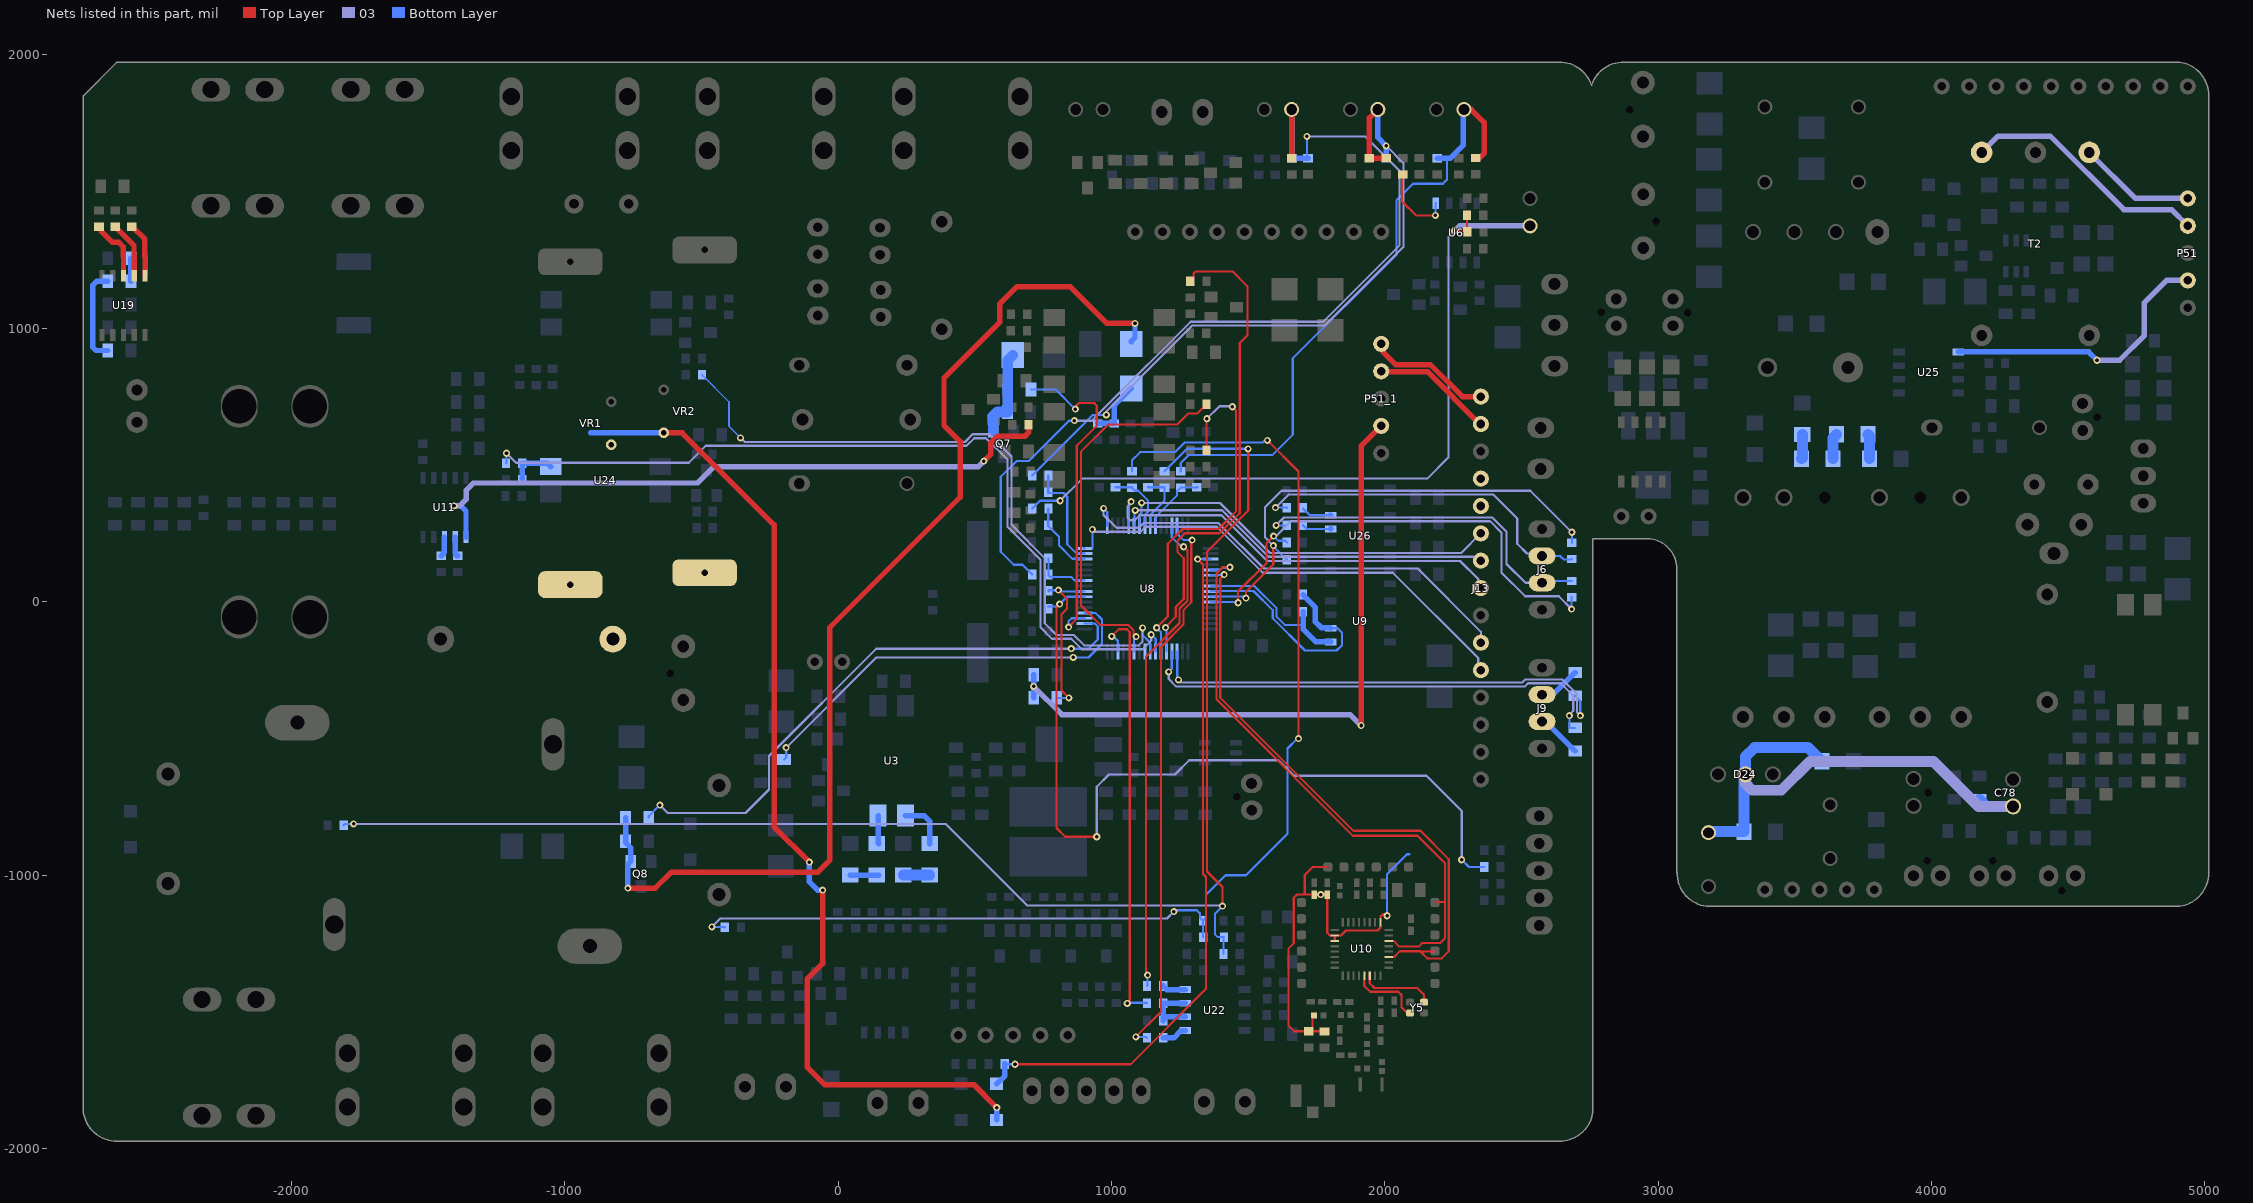
[diagram p0: the nets of this part, all layers, seen from the top]
# Altium PCB MISC105418.PcbDoc (part 6 of 7)
Units mil, origin at the board's own origin, x right, y up, seen from the top; angles counter-clockwise.
Board outline 7774.32 x 3947.04 mil, 4 copper layers (Top Layer, 02, 03, Bottom Layer), stack 30.635 mil thick; 459 components, 285 nets, 1258 pads, 468 vias.
Unrouted connection lines stored in the file: 23.

## Via types
v1: diameter 26, hole 13, Top Layer to Bottom Layer, tented both sides, 468 vias

## Nets (pads, with @x,y where several pads share a name; then routed paths per layer and width w, separated by ;. In a path a pad name is that pad's centre, name@x,y a point inside that pad or via, vN(x,y) a via of type N, cw(c..) or ccw(c..) an arc to the next point about the centre after c; other vN are vias at no path point) (continued)
NetR133_1: R133.1 R134.2 U24.4 | length 169.5
  Bottom Layer w20: R133.1@-1155.8,446.23 R134.2@-1155.8,506.5 -1064.07,506.5 U24.4@-1051.69,494.12
NetR141_1: R141.1 U26.14 | length 113.3
  Bottom Layer w8: R141.1@1700.82,340.84 1725.96,315.7 U26.14@1801.83,315.7
  Bottom Layer w20: U26.14@1800.53,317 U26.14@1801.83,315.7
NetR142_1: R142.1 U26.13 | length 107.3
  Bottom Layer w8: R142.1@1700.82,279.92 1715.03,265.7 U26.13@1801.83,265.7
  Bottom Layer w20: U26.13@1801.53,266 U26.13@1801.83,265.7
NetR147_1: R147.1 U19.8 | length 231.6
  Top Layer w19.68: R147.1@-2704,1371.04 -2701.44,1371.04 -2696.12,1365.72 -2696.12,1355.12 -2655,1314 -2631,1314 -2615,1298 -2615,1264.27
  Top Layer w20: -2615,1264.27 -2614,1263.27 U19.8@-2614,1192.27
NetR148_1: R148.1 R149.2 | length 93.9
  Bottom Layer w40: R148.1@3639.65,523.35 3639.65,599.21 R149.2@3652.44,612
NetR148_2: R148.2 R201.1 | length 89.1
  Bottom Layer w40: R148.2@3524.54,523.35 3526.98,525.79 R201.1@3526.98,611.44
NetR149_1: R149.1 R191.2 | length 91.1
  Bottom Layer w40: R149.1@3767.56,612 3773.44,606.12 R191.2@3773.44,523.35
NetR162_1: R162.1 U11.8 | length 74.5
  Bottom Layer w20: R162.1@-1451.91,168.23 -1449.35,168.23 -1444.19,173.39 -1444.19,175.94 -1439.91,180.23 U11.8@-1439.91,236.24
NetR173_2: R173.2 R175.2 U22.2 U22.3 | length 230
  Bottom Layer w20: U22.2@1269.53,-1518.96 1202.31,-1518.96 R173.2@1188.98,-1532.29 R175.2@1188.98,-1468.96 U22.3@1269.53,-1468.96
NetR174_2: R174.2 U22.1 | length 91.6
  Bottom Layer w20: R174.2@1188.98,-1595.63 1228.37,-1595.63 1255.04,-1568.96 U22.1@1269.53,-1568.96
NetR177_2: R177.2 U22.4 | length 86.1
  Bottom Layer w20: R177.2@1188.98,-1405.63 1202.31,-1418.96 U22.4@1269.53,-1418.96
NetR180_1: R180.1 U6.1 | length 287.2
  Top Layer w8: R180.1@2065,1562.28 2063,1560.28 2063,1464 2114,1413 v1(2185,1413)
  Bottom Layer w8: v1(2185,1413) 2185,1456.4 U6.1@2186.09,1457.5
NetR185_1: R185.1 R186.2 | length 84.2
  Bottom Layer w20: R186.2@-2586.91,1171.42 R185.1@-2586.91,1255.67
NetR186_1: R186.1 R187.2 | length 348
  Bottom Layer w20: R187.2@-2671.55,918.67 -2714.67,918.67 -2727,931 -2727,1157 -2712.58,1171.42 R186.1@-2671.55,1171.42
NetR189_2: R189.2 U19.6 | length 200.5
  Top Layer w20: R189.2@-2584,1371.04 -2581.44,1371.04 -2536.26,1325.86 -2536.26,1264.27 -2535.26,1263.27 U19.6@-2535.26,1192.27
NetR190_2: R190.2 U19.7 | length 209
  Top Layer w19.68: R190.2@-2644,1371.04 -2641.44,1371.04 -2636.12,1365.72 -2636.12,1363.16 -2575.63,1302.67 -2575.63,1264.27 -2574.63,1263.27 U19.7@-2574.63,1192.27
NetR195_1: R195.1 R263.1 | length 96.7
  Bottom Layer w40: R263.1@238.43,-1000.56 R195.1@335.09,-1000.56
NetR195_2: R195.2 U3.1 | length 180
  Bottom Layer w20: U3.1@246.09,-782.28 246.81,-783 315,-783 335.09,-803.09 R195.2@335.09,-885.44
NetR198_1: R198.1 U3.2 | length 103.9
  Bottom Layer w20: U3.2@146.09,-782.28 146.09,-883.54 R198.1@148,-885.44
NetR198_2: R198.2 R200.1 | length 102.9
  Bottom Layer w20: R200.1@45.09,-1000.56 R198.2@148,-1000.56
NetR264_2: R264.2 U11.7 | length 73.1
  Bottom Layer w20: U11.7@-1400.54,236.24 -1400.54,176.86 -1399.62,175.94 -1399.62,173.39 -1394.46,168.23 R264.2@-1391.91,168.23
NetU10_29: U10.29 Y5.1 | length 271.3
  Top Layer w8: U10.29@1924.94,-1368.92 1924.94,-1405.94 1946,-1427 2049,-1427 2061,-1439 2061,-1484 2081.58,-1504.58 Y5.1@2091.99,-1504.58
NetU10_30: U10.30 Y5.3 | length 269.9
  Top Layer w8: U10.30@1944.62,-1368.92 1944.62,-1395.62 1962,-1413 2118,-1413 2143.17,-1438.17 Y5.3@2143.17,-1465.21
NetVR1_1: VR1.1 VR2.2 ZC1.2
NTC-GUN: C117.2 J1.1 R150.1 R151.1 | length 2283.1
  Top Layer w20: J1.1@2289.09,1800.5 2315.5,1800.5 2363,1753 2363,1640 2345.91,1622.91 C117.2@2332,1622.91
  Bottom Layer w8: R151.1@1253.32,476.54 1253.32,507.32 1282,536 1588,536 1663,611 1663,890 2043,1270 2043,1469 2103,1529 2212,1529 2218.77,1536 2226.39,1543.61 2227.23,1544.23 2227.23,1621.72
  Bottom Layer w20: R150.1@2191.62,1621.72 2238.72,1621.72 2287,1670 2287,1798.41 J1.1@2289.09,1800.5
NTC-GUN-ADC-PB0: C116.1 R151.2 U8.26 | length 238.6
  Bottom Layer w8: U8.26@1161.62,277.82 1161.62,310.62 1240,389 1240,403.77 R151.2@1253.32,417.09 1310.39,417.09 C116.1@1311.57,418.28 C116.1@1314.13,418.28
NTC-PLUG: C66.1 J2.1 R152.1 R153.1 | length 2828.1
  Top Layer w8: v1(2255.36,1356.64) 2298.43,1356.64 R152.1@2300.46,1354.6 ; C66.1@2300.46,1413.53 R152.1@2300.46,1354.6 ; R152.1@2301.65,1353.42 R152.1@2300.46,1354.6
  03 w8: v1(812,369) 893,450 2155.17,450 2233,527.83 2233,1334.29 v1(2255.36,1356.64)
  03 w20: v1(2255.36,1356.64) 2273.41,1374.7 J2.1@2531.09,1374.7
  Bottom Layer w8: R153.1@710.26,340.69 738.57,369 v1(812,369)
NTC-PLUG-ADC-PA0: C65.1 R153.2 U8.14 | length 266.1
  Bottom Layer w8: R153.2@769.71,340.69 768.53,339.51 C65.1@768.53,279.08 768.53,276.52 808,237.05 808,206 856.91,157.09 900.46,157.09 U8.14@901.78,155.77
PE-CHECK: P51.4 P51_1.4 R197.2 R199.2 U25.1 | length 3511.3
  Top Layer w20: v1(1913,-453) 1913,569.04 P51_1.4@1986.72,642.76
  03 w19.68: v1(4605,883) 4688,883 4778,973 4778,1094 4859,1175 P51.4@4937,1175
  03 w20: v1(715.35,-310) 818.35,-413 1873,-413 v1(1913,-453)
  Bottom Layer w19.68: U25.1@4097.36,913.5 4574.5,913.5 v1(4605,883)
  Bottom Layer w20: R199.2@715.35,-351 v1(715.35,-310) R197.2@715.35,-267
PE-DI-PC0: C15.1 R199.1 U8.8 | length 610.3
  Top Layer w8: v1(806,42) 837,11 837,-26 817,-46 817,-325 v1(844,-352)
  Bottom Layer w8: C15.1@771.23,37.66 C15.1@768.53,40.36 770.17,42 v1(806,42) 810.34,37.66 U8.8@901.78,37.66 ; R199.1@800,-351 801,-352 v1(844,-352)
PLC+: J13.2 P51.2 P51_1.2 T2.2 | length 1358.9
  Top Layer w19.68: P51_1.2@1986.72,842.76 1988.16,841.31 2155.36,841.31 2346.98,649.7 J13.2@2351.09,649.7
  03 w19.68: T2.2@4183,1643.29 4242.71,1703 4434,1703 4703,1434 4878,1434 P51.2@4937,1375
PLC-: J13.1 P51.1 P51_1.1 T2.1 | length 888.1
  Top Layer w19.68: P51_1.1@1986.72,942.76 1994.25,935.22 1994.25,911.75 2039,867 2166,867 2283.3,749.7 J13.1@2351.09,749.7
  03 w19.68: T2.1@4576.7,1643.29 4744.99,1475 P51.1@4937,1475
Relay-12V-DO-PC15: R72.1 U8.4 | length 1521.9
  03 w8: v1(-190,-534) 140,-204 v1(860,-204)
  Bottom Layer w8: R72.1@-197.91,-577.8 -190,-569.89 v1(-190,-534) ; v1(860,-204) 915.58,-204 965,-154.58 965,-65 941.08,-41.08 U8.4@901.78,-41.08
Relay-L-DO-PC14: R67.2 U8.3 | length 1227.2
  Top Layer w8: v1(843,-93) 873,-63 873,570 946,643 946,717 936,727 880.86,727 868,714.14 v1(868,704)
  Bottom Layer w8: R67.2@705.32,776 796,776 v1(868,704) ; v1(843,-93) 843,-72 854.24,-60.76 U8.3@901.78,-60.76
Relay-N-DO-PC13: R71.2 U8.2 | length 2110.9
  03 w8: v1(-652,-744) -623,-773 -339,-773 -253,-687 -253,-564.47 139.47,-172 v1(853,-172)
  Bottom Layer w8: R71.2@-692.8,-790.06 -692.8,-784.74 -652.06,-744 v1(-652,-744) ; v1(853,-172) 916,-172 949.42,-138.58 949.42,-90.42 939.45,-80.45 U8.2@901.78,-80.45
reserve1: C71.1 J3.1 R154.1 R155.1 R156.2 | length 2552.7
  Top Layer w20: J3.1@1974.09,1800.5 1943,1769.41 R156.2@1943,1621.72 2003.82,1621.72 C71.1@2005,1622.91
  03 w8: v1(981,683) 981,695.73 985.27,700 985.33,700 1295.33,1010 1780,1010 2068,1298 2068,1604 v1(2004.81,1667.19)
  Bottom Layer w8: R155.1@710.26,461.54 931.72,683 v1(981,683)
  Bottom Layer w20: J3.1@1974.09,1800.5 1974.09,1697.91 v1(2004.81,1667.19) R154.1@2004.81,1621.72
Reserve1-ADC-PA1: C70.1 R155.2 U8.15 | length 391.8
  Bottom Layer w8: R155.2@769.71,461.54 768.53,460.36 C70.1@768.53,399.93 768.53,397.38 824.62,397.38 838,384 838,209.94 871.17,176.77 900.46,176.77 U8.15@901.78,175.46
reserve2: C77.1 J4.1 R157.1 R158.1 R159.2 | length 3399.2
  Top Layer w20: J4.1@1659.09,1800.5 1659.09,1622.44 R157.1@1659.85,1621.69
  03 w8: v1(864,662) 927.53,662 950,684.47 950,684.53 979.47,714 979.53,714 1289.53,1024 1774.2,1024 2054,1303.8 2054,1575 1927,1702 v1(1715,1702)
  Bottom Layer w8: R158.1@710.26,98.97 674.23,135 642,135 595,182 595,456.72 652.28,514 696.47,514 844.47,662 v1(864,662) ; v1(1715,1702) 1715,1629.77 1721,1623.77 C77.1@1719.09,1621.87
  Bottom Layer w20: J4.1@1659.09,1800.5 1660.28,1799.32 R159.2@1660.28,1620.69 1661.46,1621.87 C77.1@1719.09,1621.87
Reserve2-ADC-PC2: C73.1 R158.2 U8.10 | length 202.4
  Bottom Layer w8: C73.1@768.53,158.22 769.71,157.04 769.71,96.41 776.12,90 852.53,90 864.18,78.35 900.46,78.35 U8.10@901.78,77.03
RESET: C40.1 R236.2 U8.7 | length 3038.8
  Top Layer w8: v1(810,-9) 799,-20 799,-828 831,-860 v1(946,-860)
  03 w8: v1(946,-860) 946,-677 991,-632 1232,-632 1284,-580 1611,-580 1668,-637 2152,-637 2281,-766 v1(2281,-944)
  Bottom Layer w8: C40.1@768.53,-18.07 800.93,-18.07 v1(810,-9) 836.98,17.98 U8.7@901.78,17.98 ; v1(2281,-944) 2307.5,-970.5 R236.2@2363.65,-970.5
RS485-DIR3-PB9: R175.1 U8.62 | length 1584.8
  Top Layer w8: v1(1001,-127) 1026.84,-101.16 1056.64,-101.16 1067,-111.53 1067,-1460 v1(1057.74,-1469.26)
  Bottom Layer w8: v1(1001,-127) 1006.78,-127 1023.83,-144.04 U8.62@1023.83,-182.81 ; v1(1057.74,-1469.26) 1060,-1467 1127.57,-1467 R175.1@1129.53,-1468.96
RS485-DIR7-PB5: U8.57
RST: J13.5
RX1-in: J6.3 R137.2 R142.2 | length 1305.2
  03 w8: v1(1602,279) 1631,308 2393,308 2445,256 2445,138 2514.15,68.85 J6.3@2575.09,68.85
  Bottom Layer w8: v1(1602,279) 1640.45,279 R142.2@1641.37,279.92 ; J6.3@2575.09,68.85 2582.24,76 2683.52,76 R137.2@2684.09,75.43
RX4-in: J9.3 R139.2 | length 165.6
  Bottom Layer w20: J9.3@2575.09,-438.51 2588.19,-438.51 R139.2@2696,-546.32
SCL3-PA8: R54.2 U8.41 U9.6 | length 874.2
  Bottom Layer w8: U8.41@1362.41,37.66 1363.72,38.98 1392.6,38.98 ; 1392.62,39 1519.36,39 1590,-31.64 1590,-61 1708,-179 1823,-179 1843,-159 1843,-114 1826.42,-97.42 U9.6@1801.83,-97.42
  Bottom Layer w20: R54.2@1700.82,25.99 1700.82,23.43 1746,-21.75 1746,-74 1767.48,-95.48 1799.89,-95.48 U9.6@1801.83,-97.42
SDA3-PC9: R53.2 U8.40 U9.5 | length 600.1
  Bottom Layer w8: U8.40@1362.41,57.35 1522.65,57.35 1604,-24 1604,-55.2 1633.8,-85 1698.82,-85 1700.82,-87
  Bottom Layer w20: R53.2@1700.82,-37.5 1700.82,-87 1700.82,-100.82 1747.42,-147.42 U9.5@1801.83,-147.42
SET: J13.4
SPD-DI: D31.2 VR1.3 VR2.4 | length 3699.9
  Top Layer w20: VR2.4@-638,617.52 -570.52,617.52 -234,281 -234,-824 v1(-105,-953) ; v1(-57,-1055) -57,-1324 -113,-1380 -113,-1702.94 -48.94,-1767 496.14,-1767 v1(580.14,-1851)
  Bottom Layer w20: -904,617.52 VR2.4@-638,617.52 ; v1(-105,-953) -105,-1025 -75,-1055 v1(-57,-1055) ; D31.2@579.98,-1895.94 580.14,-1895.78 v1(580.14,-1851)
SPD-DI-PB14: D31.1 R240.2 U8.35 | length 2568.5
  Top Layer w8: v1(647,-1692) 1070,-1692 1346,-1416 1346,-1007 1335,-996 1335,-534.77 1335.07,-534.71 1335.07,135.63 v1(1315,155.7)
  Bottom Layer w8: R240.2@609.7,-1690.94 610.76,-1692 v1(647,-1692) ; v1(1315,155.7) U8.35@1362.37,155.74 ; U8.35@1362.37,155.74 U8.35@1362.41,155.77
  Bottom Layer w20: D31.1@579.98,-1764.06 609.7,-1734.33 R240.2@609.7,-1690.94
SPI-CLK-PA5: J13.8 U8.21 | length 1584.2
  03 w8: v1(1072,366) 1072,361.13 1058,347.13 1058,308 1068,298 1085,298 1103,316 1402.4,316 1569.4,149 2275,149 2341.33,82.67 2341.33,59.46 J13.8@2351.09,49.7
  Bottom Layer w8: U8.21@1063.2,277.82 1063.2,357.2 v1(1072,366)
SPI-MISO-PA6: J13.7 U8.22 | length 1398.3
  03 w8: v1(1087,334) 1404.2,334 1574.2,164 2322.98,164 2337.28,149.7 J13.7@2351.09,149.7
  Bottom Layer w8: U8.22@1082.88,277.82 1084.2,279.13 1084.2,331.2 v1(1087,334)
SPI-MOSI-PA7: J13.6 U8.23 | length 1432.9
  03 w8: v1(1110,361) 1396.99,361 1579.99,178 2279.39,178 J13.6@2351.09,249.7
  Bottom Layer w8: U8.23@1102.57,277.82 1102.57,317.04 1110,324.47 v1(1110,361)
STOP_L: D19.1 Q7.1 R67.1 R68.2 | length 356.4
  Bottom Layer w39.37: Q7.1@567.6,623.26 567.6,677.4 567,678 583,694 R68.2@619.68,694 620.68,695 R67.1@620.68,776 620.68,883.15 D19.1@639.2,901.67 D19.1@620.58,883.05
STOP_N: D6.1 Q8.1 R71.1 R74.2 | length 4040.3
  Top Layer w19.68: v1(-769,-1048) -669,-1048 -611,-990 -75,-990 -30.2,-945.2 -30.2,-415.2 -30.65,-414.76 -30.65,-94.96 446.16,381.85 446.16,586.15 387.5,644.81 387.5,817.5 591,1021 591,1088 655,1152 849,1152 983,1018 v1(1086,1018)
  Bottom Layer w19.68: R71.1@-777.44,-790.06 R74.2@-777.44,-876.15 -777.44,-881.46 -758.74,-900.17 Q8.1@-758.74,-949.89 -769,-960.15 v1(-769,-1048) ; D6.1@1071.8,951.35 1086,965.54 v1(1086,1018)
Switch-OFF: D10.1 R41.2 R238.2 | length 213.7
  Bottom Layer w20: R41.2@950.04,651.72 R238.2@1009.7,651.72 1010,652.02 1010,718.2 D10.1@1071.8,780
TEMP-Board: C58.2 R118.1 R119.1 RNTC2.2 | length 5654
  Top Layer w8: v1(1406,-1114) 1406,-1044 1349.07,-987.07 1349.07,-812.3 1349,-812.23 1349,-540.57 1349.07,-540.51 1349.07,182.55 1500,333.48 v1(1500,559)
  03 w8: v1(-1772,-813) 393,-813 691,-1111 1403,-1111 v1(1406,-1114)
  Bottom Layer w8: RNTC2.2@-1808.28,-818 -1803.28,-813 v1(-1772,-813) ; R119.1@1193.89,476.54 1276.35,559 v1(1500,559) ; v1(1406,-1114) 1379,-1141 1379,-1218 1388.17,-1227.17 R118.1@1411.18,-1227.17 1410,-1228.35 C58.2@1410,-1289.07
TEMP-Board-ADC-PC5: C57.1 R119.2 U8.25 | length 221.9
  Bottom Layer w8: C57.1@1133.29,418.28 1192.71,418.28 R119.2@1193.89,417.09 1193.89,368.77 1141.94,316.81 U8.25@1141.94,277.82
TEMP-RL: C56.2 R115.1 R116.1 RNTC1.2 | length 4517.5
  Top Layer w8: v1(1570,590) 1684,476 v1(1684,-501) ; v1@1678,-502 v1@1678,-501
  03 w8: v1(-462,-1190) -431,-1159 1203,-1159 v1(1228,-1134)
  Bottom Layer w8: v1(-462,-1190) -415.72,-1190 RNTC1.2@-414.72,-1191 ; R116.1@1075.04,476.54 1075.04,517.04 1105,547 1232.5,547 1267.5,582 1553,582 1561,590 v1(1570,590) ; v1(1228,-1134) 1233,-1129 1312,-1129 1324,-1141 1324,-1156.72 C56.2@1334.9,-1167.62 ; R115.1@1336.08,-1227.17 1334.9,-1225.99 C56.2@1334.9,-1167.62 ; v1(1684,-501) 1680,-501 1644,-537 1644,-849 1492,-1001 1417,-1001 1346,-1072 1346,-1156.52 C56.2@1334.9,-1167.62
TEMP-RL-ADC-PC4: C55.1 R116.2 U8.24 | length 235.5
  Bottom Layer w8: C55.1@1014.43,418.28 1073.86,418.28 R116.2@1075.04,417.09 1086.2,405.94 1097.59,405.94 1133,370.53 1133,327.67 1122.25,316.93 U8.24@1122.25,277.82
TL_VDD: C123.1 C124.1 C125.1 FB2.2 R42.1 U10.9 U10.18 U10.19 | length 1716.4
  Top Layer w8: R42.1@1741.51,-1513.58 1735,-1520.09 1735,-1557.87 C125.1@1721.09,-1571.77 ; FB2.2@1779.09,-1572.77 1778.09,-1571.77 C125.1@1721.09,-1571.77 ; 1791.19,-971 1736,-971 1707,-1000 1707,-1071 1707.49,-1071.49 C123.1@1741.73,-1071.49 ; U10.19@1816.67,-1240.97 U10.18@1816.67,-1221.28 ; v1(2008,-1149) 2002,-1143 1993,-1143 1983.99,-1152.01 U10.9@1983.99,-1172.07 1983.99,-1192 1972.99,-1203 1858,-1203 1839.72,-1221.28 U10.18@1816.67,-1221.28 ; C125.1@1721.09,-1571.77 1668.62,-1571.77 1647,-1550.15 1647,-1270 1667,-1250 1667,-1083 1678.51,-1071.49 C123.1@1741.73,-1071.49 ; C123.1@1741.73,-1071.49 C124.1@1789.02,-1071.49 1789.02,-1210.92 1799.38,-1221.28 U10.18@1816.67,-1221.28
  Bottom Layer w8: v1(2008,-1149) 2008,-997 2081,-924 2089,-924
  other v1: 1765.37,-1071.49
TX1-out: J6.2 R141.2 R170.2 | length 1314.6
  03 w8: v1(1600,344) 1648,392 2396,392 2484,304 2484,212 2520.11,175.89 2566.48,175.89 J6.2@2575.09,167.28
  Bottom Layer w8: v1(1600,344) 1640.77,344 R141.2@1641.37,343.4 ; J6.2@2575.09,167.28 2640.72,167.28 2654,154 2681.84,154 R170.2@2684.09,156.25
  Bottom Layer w20: J6.2@2575.09,167.28 J6.2@2586.12,156.25
TX4-out: J9.2 R140.2 | length 160.3
  Bottom Layer w20: J9.2@2579.31,-344.3 J9.2@2575.09,-340.09 2615.73,-340.09 R140.2@2696.16,-259.65
UT1-RX-PA10: R18.1 R137.1 U8.43 | length 1831.8
  Top Layer w8: v1(1463,-4) 1463,37 1567,141 1567,214 v1(1593,240)
  03 w8: v1(1593,240) 1603,240 1657,294 2385,294 2427,252 2427,106 2513,20 2636,20 v1(2683,-27)
  Bottom Layer w8: U8.43@1362.41,-1.71 1460.71,-1.71 v1(1463,-4) ; v1(1593,240) 1610.5,222.5 1635.3,222.5 R18.1@1641.37,216.43 ; v1(2683,-27) 2683,14.88 R137.1@2684.09,15.98
UT1-TX-PA9: R83.1 R170.1 U8.42 | length 1840
  Top Layer w8: v1(1492,13) 1492,36 1592,136 v1(1592,205)
  03 w8: v1(1592,205) 1562,235 1562,346 1622,406 2532,406 v1(2684,254)
  Bottom Layer w8: U8.42@1362.41,17.98 1363.43,19 1486,19 v1(1492,13) ; v1(1592,205) 1592,202.32 R83.1@1641.37,152.95 ; v1(2684,254) 2684,215.8 R170.1@2684.09,215.7
UT2-RX/SPI-\R\S\T\-PA3: J13.10 U8.17 | length 1704.9
  03 w8: v1(971,341) 971,317 1018,270 1100.8,270 1118.8,288 1390.8,288 1557.8,121 2120,121 2351.09,-110.09 J13.10@2351.09,-150.3
  Bottom Layer w8: v1(971,341) 984.46,327.54 U8.17@984.46,277.82
UT2-TX/SPI-\I\N\T\-PA2: J13.11 U8.16 | length 1743.4
  03 w8: v1(930,264) 938,256 1106.6,256 1124.6,274 1385,274 1553,106 2029,106 2341.33,-206.33 2341.33,-240.53 J13.11@2351.09,-250.3
  Bottom Layer w8: U8.16@898,196.46 899.32,195.14 U8.16@901.78,195.14 ; U8.16@930,194 v1(930,264)
UT3-RX-PB11: R174.1 U8.30 | length 2038
  Top Layer w8: v1(1089,-1592) 1181,-1500 1181,-165.8 1263,-83.8 1263,-31 1292,-2 1292,222 v1(1295,225)
  Bottom Layer w8: v1(1089,-1592) 1125.9,-1592 R174.1@1129.53,-1595.63 ; U8.30@1240.36,277.82 1241.68,276.5 1241.68,247.2 1263.88,225 v1(1295,225)
UT3-TX-PB10: R177.1 U8.29 | length 1780.6
  Top Layer w8: v1(1132,-1366) 1126.69,-1360.69 1126.69,-200.31 1249,-78 1249,-25.2 1278,3.8 1278,187 v1(1264,201)
  Bottom Layer w8: R177.1@1129.53,-1405.63 1132,-1403.16 v1(1132,-1366) ; U8.29@1220.68,277.82 1220.68,235.68 1258.35,198 1261.35,201 v1(1264,201)
UT4-RX-PC11: R139.1 U8.52 | length 1769
  03 w8: v1(1209.13,-257.13) 1209.13,-282.81 1237.1,-310.77 2511.23,-310.77 2523.41,-298.59 2643.59,-298.59 2689.4,-344.4 2689.4,-399.6 v1@2675,-414 ; v1(2675,-417) v1@2675,-414 ; v1@2679,-418 v1@2675,-414
  Bottom Layer w8: v1(1209.13,-257.13) 1220.68,-245.59 U8.52@1220.68,-182.81 ; v1(2675,-417) 2675,-459 2677.68,-461.68 R139.1@2696,-461.68
UT4-TX-PC10: R140.1 U8.51 | length 1758.5
  03 w8: v1(1245.09,-286.23) 1254.86,-296 2502,-296 2513.41,-284.59 2649.39,-284.59 2703.4,-338.6 2703.4,-405.4 v1(2715,-417)
  Bottom Layer w8: U8.51@1240.36,-182.81 1240.36,-281.51 v1(1245.09,-286.23) ; R140.1@2696.16,-344.3 2715,-363.14 v1(2715,-417)
UT5-EL-RX: R87.1 U8.54 | length 1333.6
  Top Layer w8: v1(1164.88,-95.35) 1206,-54.23 1206,212 1260,266 1391.6,266 1455,329.4 1455,700 v1(1442,713) ; R87.1@1347.83,554 1347.83,667.83 v1(1349,669)
  03 w8: v1(1349,669) 1395,715 1440,715 v1(1442,713)
  Bottom Layer w8: v1(1164.88,-95.35) 1181.31,-111.78 U8.54@1181.31,-182.81
UT5-EL-TX: R65.1 U8.53 | length 1811.5
  Top Layer w8: v1(1198,-95) 1198,-92.76 1235,-55.76 1235,-19.4 1264,9.6 1264,159.03 1241,182.03 1241,222 1269,250 1395.4,250 1469,323.6 1469,945.8 1497,973.8 1497,1154 1442.84,1208.16 1309.16,1208.16 1299.54,1198.54 1299.54,1183.06 R65.1@1288.38,1171.91
  Bottom Layer w8: v1@1196.99,-94.07 1200.99,-98.07 U8.53@1200.99,-182.81
UT6-BLE-RX: U8.38 U10.3 | length 2225.8
  Top Layer w8: v1(1412,98.72) 1398.07,84.78 1398.07,-351.2 1884.87,-838 2130.2,-838 2234,-941.8 2234,-1278.84 2208,-1304.84 2155,-1304.84 2130.16,-1280 2183,-1280 ; U10.3@2013.52,-1300.02 2033.98,-1300.02 2055,-1279 2129.16,-1279
  Bottom Layer w8: U8.38@1362.41,96.72 1363.41,97.72 1411,97.72 v1(1412,98.72)
UT6-BLE-TX: U8.37 U10.6 | length 2225.3
  Top Layer w8: v1@1443,126 v1(1433,126) 1406.76,126 1384.07,103.31 1384.07,-357 1883.07,-856 2119.53,-856 2220,-956.47 2220,-1099 ; U10.6@2013.52,-1240.97 2032,-1240.97 2053.03,-1262 2123.79,-1262 2136.79,-1249 2202.79,-1249 2220,-1231.79 2220,-1099 ; 2187,-1099 2220,-1099
  Bottom Layer w8: U8.37@1363.72,117.72 U8.37@1362.41,116.4 1397.16,116.4 1406.76,126 v1(1433,126)
UT7-RX-PB3: R134.1 U8.55 | length 3160.1
  03 w8: v1(-1213,543) -1178,508 -546,508 -484,570 469.72,570 497.72,598 541,598 620,519 620,273 740,153 740,-94 782,-136 853,-136 891,-174 1114,-174 1145.32,-142.68 v1@1145.32,-120.68
  Bottom Layer w8: R134.1@-1215.25,506.5 -1213,508.75 v1(-1213,543) ; v1(1145,-121) 1145.64,-121 1161.62,-136.98 U8.55@1161.62,-182.81
UT7-TX-PB4: R109.1 U8.56 | length 2538.1
  03 w8: v1(-357,599) -342,584 463.92,584 491.92,612 553.28,612 634,531.28 634,281 756,159 756,-79 799,-122 862,-122 900,-160 1100,-160 1114,-146 v1(1114,-96)
  Bottom Layer w6: R109.1@-498.12,829.5 -399,730.38 -399,641.59 -357,599.59 v1(-357,599)
  Bottom Layer w8: v1(1114,-96) 1114,-122.53 1135.47,-144 1136.11,-144 1140.62,-148.51 1140.62,-181.5 U8.56@1141.94,-182.81
Vout1: C78.1 C81.2 D24.2 L24.1 R22.2 R23.2 | length 1990.6
  03 w40: D24.2@3319.09,-631.5 3319.09,-665.09 3344,-690 3450,-690 3555,-585 4007,-585 4170.92,-748.92 C78.1@4298.09,-748.92
  Bottom Layer w40: L24.1@3184.09,-845.07 3187.67,-841.5 R22.2@3313.54,-841.5 3313.54,-637.06 D24.2@3319.09,-631.5 3319.09,-566.79 3352.88,-533 3547.54,-533 R23.2@3598.54,-584 ; C81.2@4175.09,-722.82 4201.2,-748.92 C78.1@4298.09,-748.92
ZX-V: R91.2 U11.6 | length 2431.2
  Top Layer w20: v1(533,514) 558,539 558,580 583,605 683,605 696.72,618.72 R91.2@696.72,647
  03 w20: v1(-1405,350) -1404.59,350.41 -1384.59,350.41 -1361,374 -1361,407 -1334.03,433.97 -514.26,433.97 -453.96,494.27 513.27,494.27 v1(533,514)
  Bottom Layer w20: v1(-1405,350) -1380,350 -1361.17,331.17 U11.6@-1361.17,236.24
ZX-V-PB7: R93.1 U8.59 | length 1408.7
  Top Layer w8: v1(1090,-127.63) 1081,-118.63 1081,-105.73 1060.27,-85 959,-85 888.38,-14.38 888.38,320.38 888,320.76 888,548 988,648 1241,648 1281,688 1313.83,688 R93.1@1347.83,722
  Bottom Layer w8: U8.59@1082.88,-182.81 1082.88,-134.75 v1(1090,-127.63)
pads on no net: ?.12 ANT1.2 C6.0 C13.0 C14.0 C36.0 C42.0 C43.0 C47.0 C78.0 C83.0 C84.0 C85.0 C121.0 D24.3 J13.3 J13.15 J50.2 J50.4 J50.6 J50.8 J50.10 J50_1.2 J50_1.4 J50_1.6 J50_1.8 J50_1.10 J55.5 J55_1.5 P51.3 P51.5 P51_1.3 P51_1.5 Q2.0 T1.2 T1.4 T1.7 T1.8 T2.5 U6.5 U10.1 U10.2 U10.4 U10.5 U10.14 U10.17 U10.20 U10.21 U10.22 U10.23 U10.24 U10.31 U10.32 U13.3 U25.5 U25.6 U25.7 U26.7 U26.8 U26.9 U26.10
copper on no net: | length 2670.9
  Top Layer w8: 1693.35,-1220.35 1773.02,-1300.02 1816.67,-1300.02 1802.02,-1300.02 ; 1694.65,-1339.39 1799.61,-1339.39 1816.67,-1339.39 ; 1694.65,-1278.11 1720.5,-1278.11 1762.09,-1319.71 1816.67,-1319.71 ; 1694.65,-1160 1710.39,-1160 1723,-1172.61 1723,-1177 1723,-1228 1734,-1239 1775.34,-1280.34 1816.67,-1280.34 ; 1704,-1102 1723,-1102 1737,-1116 1737,-1218 1755,-1236 1779.65,-1260.65 1816.67,-1260.65 ; v1(1816,-1167) 1816.67,-1167.67 1816.67,-1201.6 ; 1850.24,-970.94 1850.24,-932.76 v1(1851,-932) ; v1(1882,-1133) 1885.57,-1136.57 1885.57,-1172.07 ; v1(1959,-1281) 1959.66,-1280.34 2013.52,-1280.34 ; v1(1969,-1245) 1984.65,-1260.65 2013.52,-1260.65 ; 1983.99,-1368.92 1984.56,-1369.49 2114.49,-1369.49 2144,-1399 2183,-1399 ; 2013.52,-1319.71 2085.71,-1319.71 2094,-1328 2102,-1336 2183,-1336 ; v1(2022,-918) 2022,-965.54 2027.41,-970.94 ; 2086.46,-970.94 2086.46,-926.54 v1(2089,-924) ; v1(2142,-1160) 2183,-1160 ; v1(2144,-1218) 2145.06,-1219.06 2183,-1219.06
  Bottom Layer w8: v1(1816,-1167) 1816,-1145 1851,-1110 v1(1851,-932) ; v1(1882,-1133) 1882,-964 1910,-936 1928,-918 v1(2022,-918) ; v1(1959,-1281) 2081,-1281 v1(2144,-1218) ; v1(1969,-1245) 2070,-1245 2142,-1173 v1(2142,-1160)

## Polygon pours and split planes (outlines as drawn)
EARTH on Bottom Layer "EARTH_L04_P329" (solid, remove dead copper, pour order 329): -2082,-1921 -2379,-1921 -2409,-1891 -2409,-1444 -2370,-1405 -2090,-1405 -2059,-1436 -2059,-1898
N2 on Bottom Layer "N2_L04_P321" (solid, remove dead copper, pour order 321): -317,1195 -317,794 -253,730 362,730 530,898 530,997 620.17,1087.17 1599.17,1087.17 1732,1220 1732,1387 1713.62,1405.38 1663.38,1405.38 1644,1386 1644.01,1248.01 1544,1148 569,1148 461,1040 461,937.5 322.5,799 -212,799 -238,825 -238,1266.09 -169,1335.09 -169,1473 -308,1473 -394,1387 -394,1272
L-PLC on Bottom Layer "L-PLC_L04_P319" (solid, remove dead copper, pour order 319): -64.5,1119 -8,1062.5 -8,966 40,918 203,918 326,1041 326,1089 437,1200 1456,1200 1535,1279 1535,1381 1512,1404 1464.15,1404 1444,1383.85 1444,1306 1402,1264 413,1264 266,1117 266,1062 180,976 114,976 74,1016 74,1125 -1,1200 -119.91,1200 -135.91,1184 -135.9,1129.91 -125,1119
- on Bottom Layer "-_L04_P281" (solid, remove dead copper, pour order 281): 1262,166 1262,-46 1234,-74 1005,-74 973,-42 973,179 989.14,195.14 1237.02,195.14
N-3 on Bottom Layer "N-3_L04_P252" (solid, remove dead copper, pour order 252): 4174,1768 4280,1874 4280,1912 4267,1925 4213,1925 4200,1912 4200,1885 4124,1809 3912.99,1809 3861.05,1860.95 3704.94,1860.94 3683,1839 3683,1787 3702,1768
NetC36_1 on Bottom Layer "NETC36_1_L04_P244" (solid, remove dead copper, pour order 244): 3243,1701 3026,1701 2984,1659 2924,1659 2904,1679 2904,1731 2924,1751 3099,1751 3146,1798 3243,1798 3251,1790 3251,1709
12VA on Bottom Layer "12VA_L04_P240" (solid, remove dead copper, pour order 240): 2933,1447 2975,1447 3098,1570 3231.8,1570 3246,1584.2 3246,1648 3228,1666 3068,1666 2936,1534 2903,1501 2903,1477
L1 on Bottom Layer "L1_L04_P230" (solid, remove dead copper, pour order 230): 3471,1296 3447,1320 3447,1410 3334,1523 3334,1605 3354,1625 3603,1625 3620,1608 3620,1494 3547,1421 3547,1320 3523,1296
ACL-IN on Bottom Layer "ACL-IN_L04_P224" (solid, remove dead copper, pour order 224): -2382,1902 -2382,1371 -2382,687 -2330,635 -2157,635 -2135,657 -2135,903 -2011,1027 -2011,1894 -2058,1941 -2343,1941